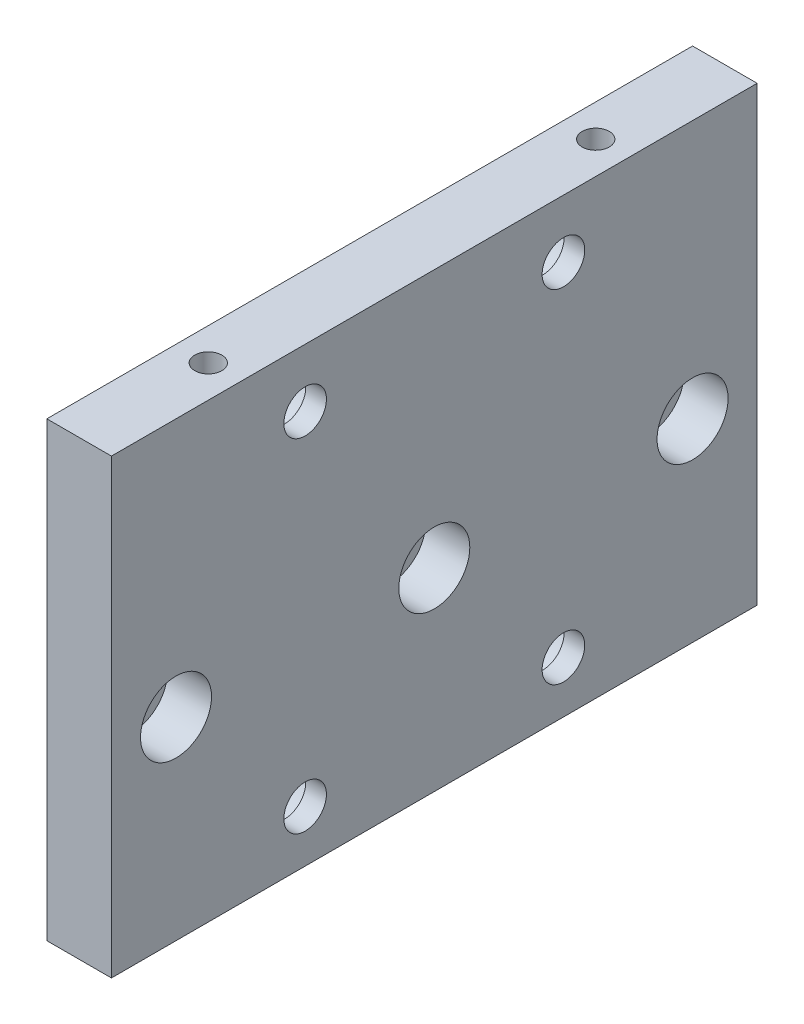
SolidWorks part; units mm, degrees
ref_plane "前视基准面" through (0, 0, 0) normal (0, 0, 1) x (1, 0, 0)
ref_plane "上视基准面" through (0, 0, 0) normal (0, 1, 0) x (1, 0, 0)
ref_plane "右视基准面" through (0, 0, 0) normal (1, 0, 0) x (0, 0, -1)
sketch "草图1" plane through (0, 0, 0) normal (1, 0, 0) x (0, 0, -1)
  line L1 (-50, 35) -> (50, 35)
  line L2 (-50, 35) -> (-50, -35)
  line L3 (-50, -35) -> (50, -35)
  line L4 (50, 35) -> (50, -35)
  line L5 (-50, 35) -> (50, -35) construction
  line L6 (-50, -35) -> (50, 35) construction
  point P0 (0, 0)
  dimension "D1" = 100
  dimension "D2" = 70
extrude "凸台-拉伸1" add sketch "草图1" along normal blind 10
hole_wizard "打孔尺寸(%根据)内六角圆柱头螺钉的类型1" positions "草图2" profile "草图3" counterbore size "M6" standard "GB"
sketch "草图2" plane through (10, 0, 0) normal (1, 0, 0) x (0, 0, -1)
  line L0 (0, 0) -> (0, -59.6587) construction
  line L2 (-50, -35) -> (50, -35) construction
  point P0 (-40, -5)
  point P2 (0, -5)
  point P4 (40, -5)
  dimension "D1" = 80
  dimension "D2" = 30
sketch "草图3" plane through (10, -5, 40) normal (0, 1, 0) x (0, 0, -1)
  line L0 (0, 0) -> (0, 16.9828)
  line L1 (0, 16.9828) -> (3.3, 15)
  line L2 (3.3, 15) -> (3.3, 6.8)
  line L3 (3.3, 6.8) -> (5.5, 6.8)
  line L4 (5.5, 6.8) -> (5.5, 0)
  line L5 (5.5, 0) -> (0, 0)
  line L10 (0, 16.9828) -> (-3.3, 15) construction
  line L11 (0, -6.35) -> (0, 107.95) construction
  dimension "孔直径" = 6.6
  dimension "孔深度" = 15
  dimension "柱形沉头孔直径" = 11
  dimension "柱形沉头孔深度" = 6.8
  dimension "导头角度" = 118
hole_wizard "打孔尺寸(%根据)内六角圆柱头螺钉的类型3" positions "草图8" profile "草图9" counterbore size "M6" standard "GB" end condition through all
sketch "草图8" plane through (0, 0, 0) normal (-1, 0, 0) x (0, 0, 1)
  line L0 (0, 34.6307) -> (0, -30.126) construction
  line L2 (50, -35) -> (-50, -35) construction
  point P0 (-20, 26)
  point P2 (20, 26)
  point P4 (-20, -27)
  point P6 (20, -27)
  dimension "D1" = 40
  dimension "D2" = 8
  dimension "D3" = 53
sketch "草图9" plane through (0, 26, -20) normal (0, 1, 0) x (0, 0, 1)
  line L0 (0, 0) -> (0, 10)
  line L1 (0, 10) -> (3.3, 10)
  line L3 (3.3, 10) -> (3.3, 6.8)
  line L4 (5.5, 6.8) -> (3.3, 6.8)
  line L5 (5.5, 6.8) -> (5.5, 0.025)
  line L6 (5.5, 0.025) -> (5.525, 0)
  line L7 (5.525, 0) -> (0, 0)
  line L8 (-5.5, 0.025) -> (-5.525, 0) construction
  line L11 (0, -6.35) -> (0, 107.95) construction
  dimension "通孔孔直径" = 6.6
  dimension "通孔孔深度" = 10
  dimension "柱形沉头孔直径" = 11
  dimension "柱形沉头孔深度" = 6.8
  dimension "近端锥形沉头孔直径" = 11.05
  dimension "近端锥形沉头孔角度" = 90
hole_wizard "M5 螺纹孔1" positions "草图10" profile "草图11" tap size "M5" standard "GB"
sketch "草图10" plane through (0, 35, 0) normal (0, 1, 0) x (1, 0, 0)
  line L0 (5, -50) -> (5, -7.7212) construction
  line L1 (10, -50) -> (0, -50) construction
  line L3 (0, 0) -> (21.3333, 0) construction
  point P0 (5, 30)
  point P2 (5, -30)
  dimension "D1" = 60
sketch "草图11" plane through (5, 35, -30) normal (1, 0, 0) x (0, 0, 1)
  line L0 (0, 0) -> (0, 13.6618)
  line L1 (0, 13.6618) -> (2.1, 12.4)
  line L2 (2.1, 12.4) -> (2.1, 0)
  line L5 (2.1, 0) -> (0, 0)
  line L10 (0, 13.6618) -> (-2.1, 12.4) construction
  line L11 (0, -6.35) -> (0, 107.95) construction
  dimension "螺纹孔钻头直径" = 4.2
  dimension "螺纹孔钻头深度" = 12.4
  dimension "导头角度" = 118
cosmetic thread "孔螺蚊线1"
cosmetic thread "孔螺蚊线2"
